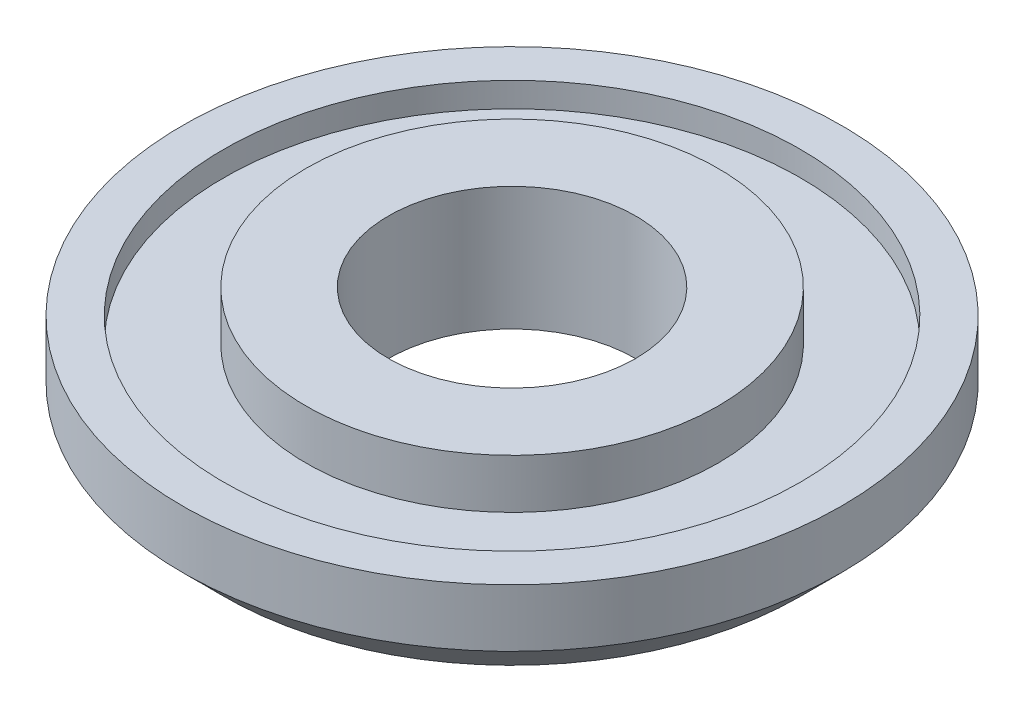
from build123d import *


with BuildPart() as part:
    # Sketch1 → Revolve1 (revolve)
    with BuildSketch(Plane.XY):
        Polygon((15, 517), (35, 517), (40, 522), (40, 529), (35, 529), (35, 526), (25, 526), (25, 532), (15, 532), align=None)
    revolve(axis=Axis((0, 517, 0), (0, 1, 0)))


solid = part.part
